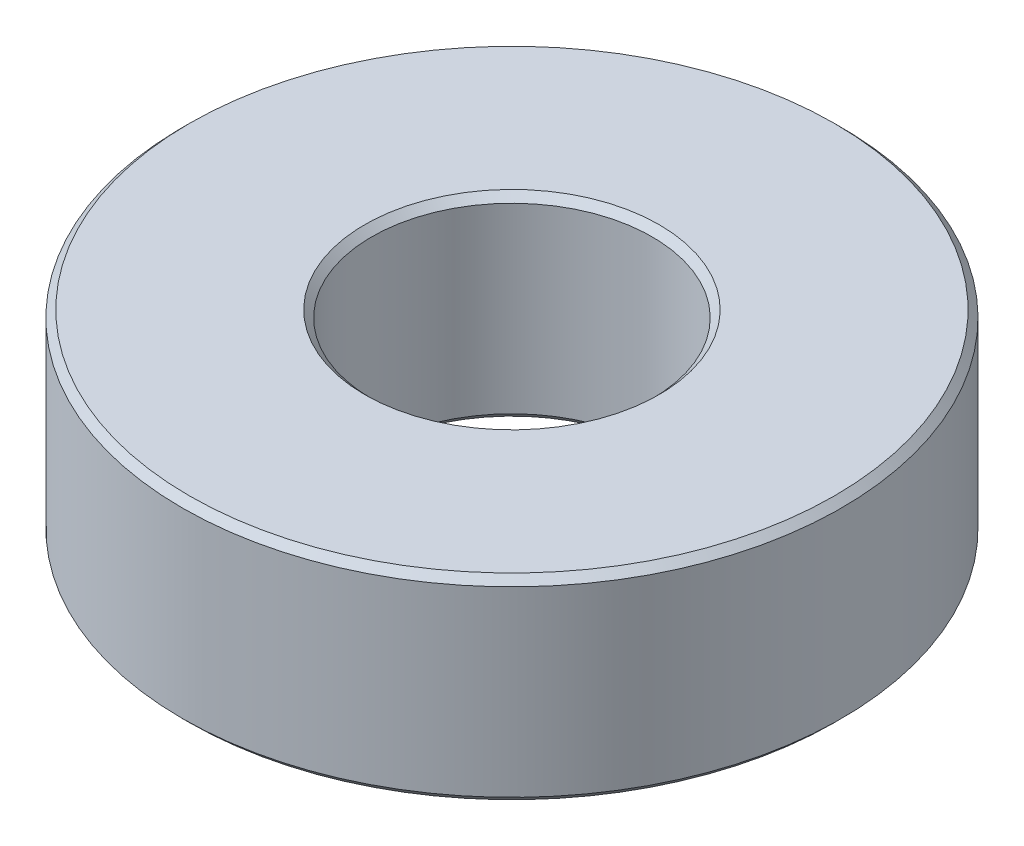
from build123d import *

# Parameters (mm, degrees)
SKETCH_1_R      = 23.5
SKETCH_1_R_2    = 10
EXTRUDE_1_DEPTH = 14
CHAMFER_1_SIZE  = 0.5


with BuildPart() as part:
    # 草图1 → 拉伸1 (new body)
    with BuildSketch(Plane(origin=(0, 0, 0), x_dir=(1, 0, 0), z_dir=(0, 1, 0))):
        with Locations(Location((0, 0, 0), (0, 0, 270))):
            Circle(SKETCH_1_R)
        with Locations(Location((0, 0, 0), (0, 0, 270))):
            Circle(SKETCH_1_R_2, mode=Mode.SUBTRACT)
    extrude(amount=EXTRUDE_1_DEPTH)

    # 倒角1
    chamfer_1_edges = [part.edges().sort_by_distance(p)[0] for p in [
        (0, 0, -23.5),
        (0, 14, -23.5),
        (0, 0, -10),
        (0, 14, -10),
    ]]
    chamfer(chamfer_1_edges, length=CHAMFER_1_SIZE)


solid = part.part
